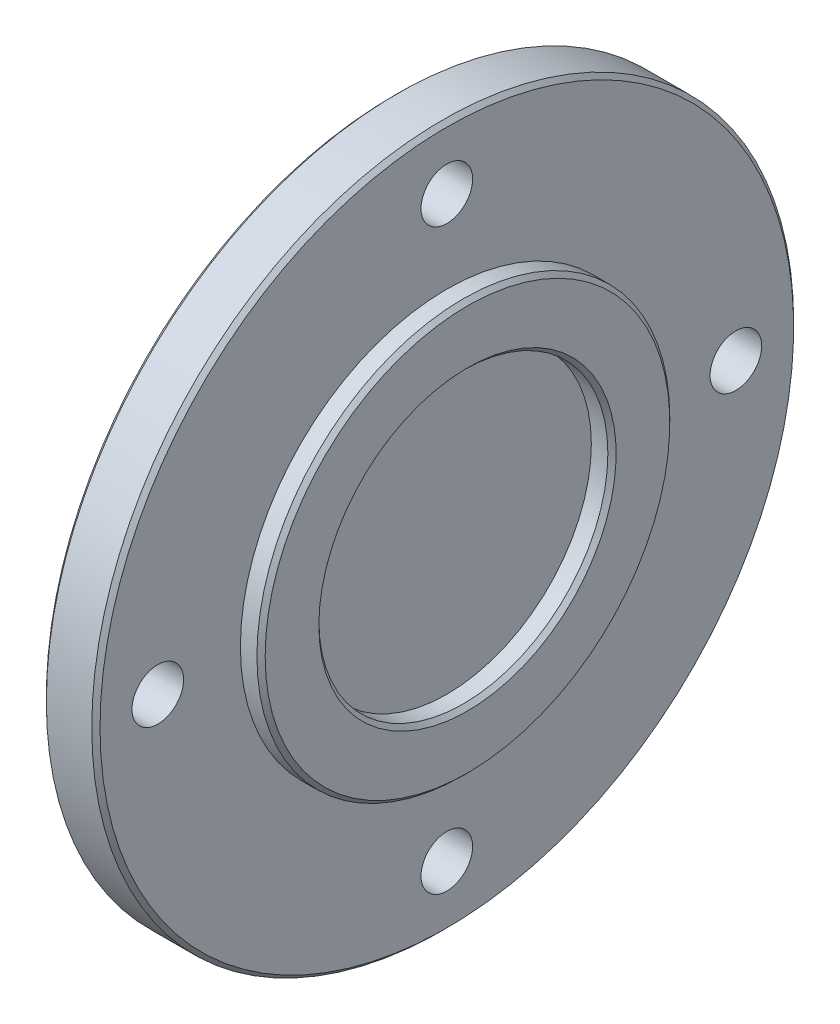
from build123d import *

# Parameters (mm, degrees)
SKETCH_2_R               = 6.25
CUT_EXTRUDE_1_DEPTH      = 122.548344291
PATTERN_CIRCULAR_1_COUNT = 4
CHAMFER_1_SIZE           = 1


with BuildPart() as part:
    # 草图1 → 旋转1 (revolve)
    with BuildSketch(Plane.XY, mode=Mode.PRIVATE) as revolve_1_sk:
        Polygon((0, 0), (0, 85), (13, 85), (13, 50), (18, 50), (18, 35), (13, 35), (13, 0), align=None)
    revolve(revolve_1_sk.sketch.rotate(Axis((0, 0, 0), (1, 0, 0)), 90), axis=Axis((0, 0, 0), (1, 0, 0)))

    # 草图2 → 切除-拉伸1 (cut, through all)
    with BuildSketch(Plane.ZY):
        with Locations((0, 70)):
            Circle(SKETCH_2_R)
    cut_extrude_1 = extrude(amount=-CUT_EXTRUDE_1_DEPTH, mode=Mode.SUBTRACT)

    # 阵列(圆周)1: 切除-拉伸1 ×4 about axis
    pattern_circular_1_axis = Axis((0, 0, 0), (1, 0, 0))
    for i in range(1, PATTERN_CIRCULAR_1_COUNT):
        add(cut_extrude_1.rotate(pattern_circular_1_axis, i * 360 / PATTERN_CIRCULAR_1_COUNT), mode=Mode.SUBTRACT)

    # 倒角1
    chamfer_1_edges = [part.edges().sort_by_distance(p)[0] for p in [
        (18, 0, -35),
        (18, 0, -50),
        (13, 0, -85),
        (0, 0, -85),
    ]]
    chamfer(chamfer_1_edges, length=CHAMFER_1_SIZE)


solid = part.part
